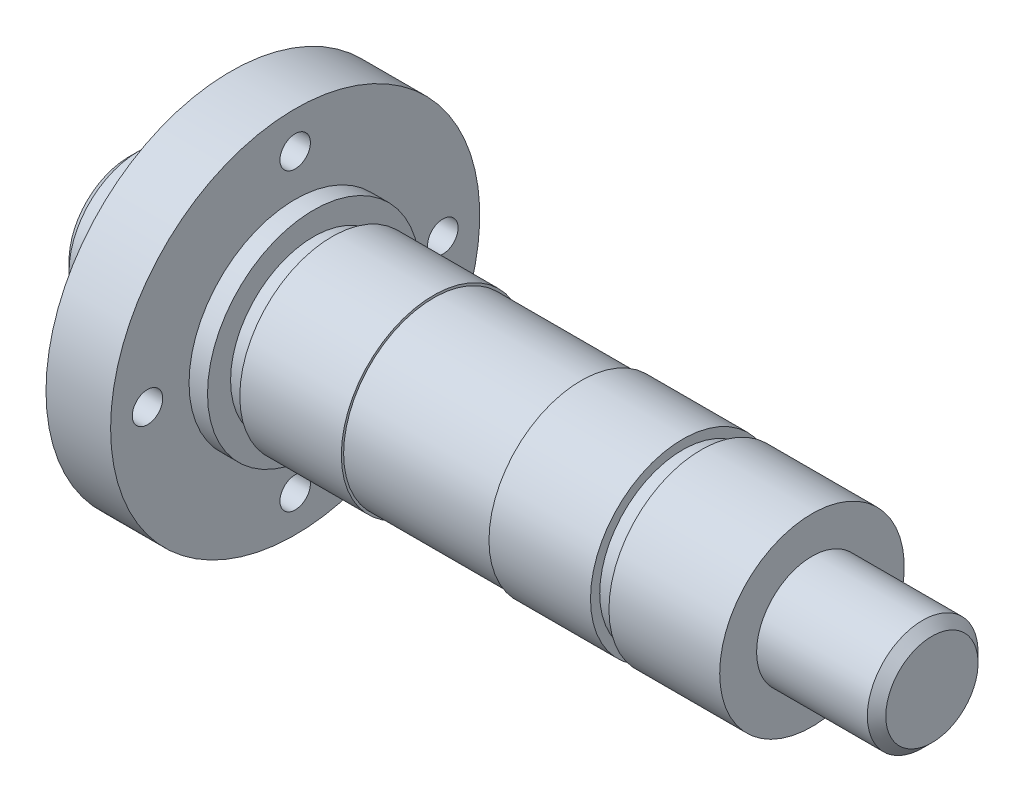
from build123d import *

# Parameters (mm, degrees)
M6_TAPPED_HOLE1_D     = 5
M6_TAPPED_HOLE1_DEPTH = 18
M6_TAPPED_HOLE1_TIP   = 1.502151548
M4_TAPPED_HOLE1_D     = 3.3
SKETCH6_W             = 2
SKETCH6_H             = 1
CHAMFER1_SIZE         = 1


with BuildPart() as part:
    # Sketch1 → Revolve1 (revolve)
    with BuildSketch(Plane.XY, mode=Mode.PRIVATE) as revolve1_sk:
        Polygon((0, 0), (87, 0), (87, 6), (74, 6), (74, 10), (62, 10), (62, 9), (60, 9), (60, 10), (49, 10), (49, 9.75), (33, 9.75), (33, 10), (20, 10), (20, 11.5), (18, 11.5), (18, 20), (11, 20), (11, 10), (8, 10), (8, 7.5), (0, 7.5), align=None)
    revolve(revolve1_sk.sketch.rotate(Axis((0, 0, 0), (1, 0, 0)), 90), axis=Axis((0, 0, 0), (1, 0, 0)))

    # M6 Tapped Hole1
    with Locations(Plane.ZY):
        with Locations((0, 0)):
            Hole(M6_TAPPED_HOLE1_D / 2, depth=M6_TAPPED_HOLE1_DEPTH)
            with Locations((0, 0, -(M6_TAPPED_HOLE1_DEPTH + M6_TAPPED_HOLE1_TIP / 2))):  # 118° drill point
                Cone(0, M6_TAPPED_HOLE1_D / 2, M6_TAPPED_HOLE1_TIP, mode=Mode.SUBTRACT)

    # M4 Tapped Hole1 (through all)
    with Locations(Plane.ZY.offset(-11)):
        with Locations((0, 16), (-16, 0), (0, -16), (16, 0)):
            Hole(M4_TAPPED_HOLE1_D / 2)

    # Sketch6 → Cut-Revolve1 (revolve, cut)
    with BuildSketch(Plane.XY, mode=Mode.PRIVATE) as cut_revolve1_sk:
        with Locations((21, 9.5)):
            Rectangle(SKETCH6_W, SKETCH6_H)
    revolve(cut_revolve1_sk.sketch.rotate(Axis((0, 0, 0), (1, 0, 0)), 90), axis=Axis((0, 0, 0), (1, 0, 0)), mode=Mode.SUBTRACT)

    # Chamfer1
    chamfer1_edges = [part.edges().sort_by_distance(p)[0] for p in [
        (87, 0, -6),
        (0, 0, -7.5),
    ]]
    chamfer(chamfer1_edges, length=CHAMFER1_SIZE)


solid = part.part
